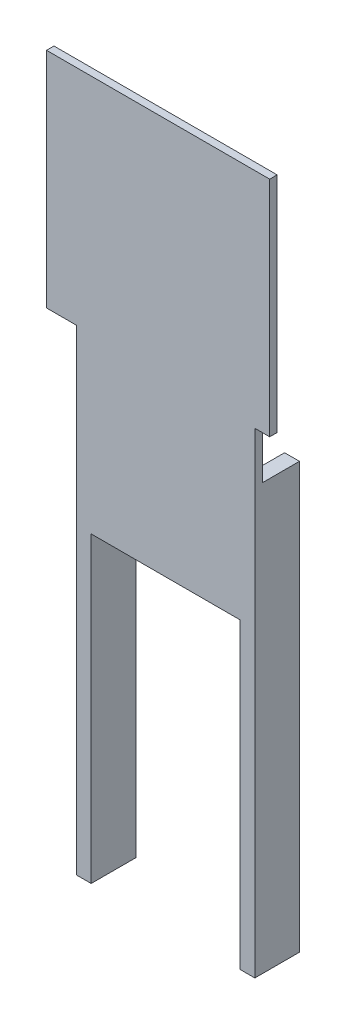
from build123d import *

# Parameters (mm, degrees)
BOSS_EXTRUDE1_DEPTH = 5
SKETCH2_W           = 10
SKETCH2_H           = 285.757818937
SKETCH2_H_2         = 313.599020197
BOSS_EXTRUDE2_DEPTH = 30
CHAMFER1_SIZE       = 3.5


with BuildPart() as part:
    # Sketch1 → Boss-Extrude1 (new body)
    with BuildSketch(Plane.XY):
        Polygon((-60, 40), (-60, -80), (60, -80), (60, 40), (70, 40), (70, 190), (-80, 190), (-80, 40), align=None)
    extrude(amount=BOSS_EXTRUDE1_DEPTH)

    # Sketch2 → Boss-Extrude2 (add)
    with BuildSketch(Plane.XY.offset(5)):
        with Locations((55, -137.121090531)):
            Rectangle(SKETCH2_W, SKETCH2_H)
        with Locations((-55, -123.200489901)):
            Rectangle(SKETCH2_W, SKETCH2_H_2)
    extrude(amount=-BOSS_EXTRUDE2_DEPTH)

    # Chamfer1
    chamfer1_edges = [part.edges().sort_by_distance(p)[0] for p in [
        (0, -80, 5),
    ]]
    chamfer(chamfer1_edges, length=CHAMFER1_SIZE)


solid = part.part
